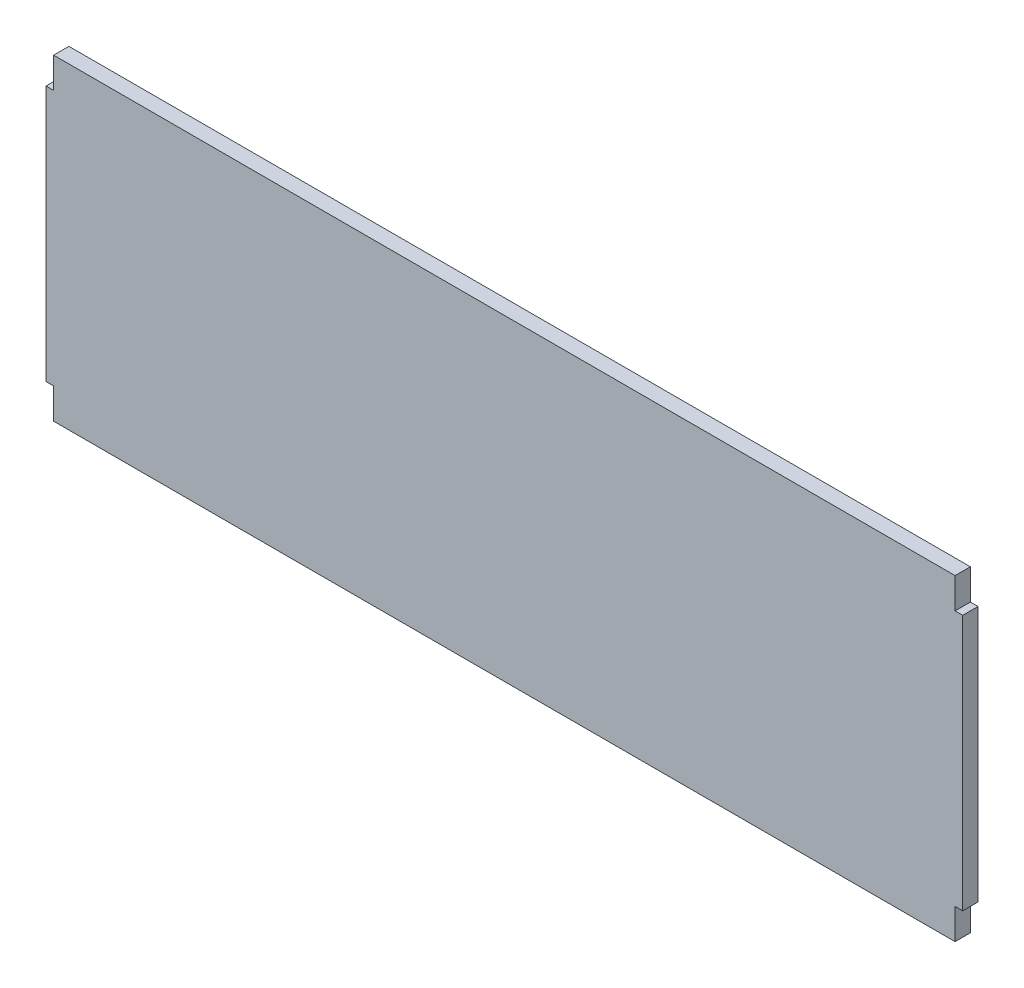
from build123d import *

# Parameters (mm, degrees)
SKETCH1_W           = 1200
SKETCH1_H           = 415
BOSS_EXTRUDE1_DEPTH = 20
SKETCH2_W           = 10
SKETCH2_H           = 40
CUT_EXTRUDE1_DEPTH  = 280


with BuildPart() as part:
    # Sketch1 → Boss-Extrude1 (new body)
    with BuildSketch(Plane.XY):
        with Locations((600, 207.5)):
            Rectangle(SKETCH1_W, SKETCH1_H)
    extrude(amount=BOSS_EXTRUDE1_DEPTH)

    # Sketch2 → Cut-Extrude1 (cut)
    with BuildSketch(Plane.XY.offset(20)):
        with Locations((5, 395)):
            Rectangle(SKETCH2_W, SKETCH2_H)
        with Locations((1195, 395)):
            Rectangle(SKETCH2_W, SKETCH2_H)
        with Locations((1195, 20)):
            Rectangle(SKETCH2_W, SKETCH2_H)
        with Locations((5, 20)):
            Rectangle(SKETCH2_W, SKETCH2_H)
    extrude(amount=-CUT_EXTRUDE1_DEPTH, mode=Mode.SUBTRACT)


solid = part.part
